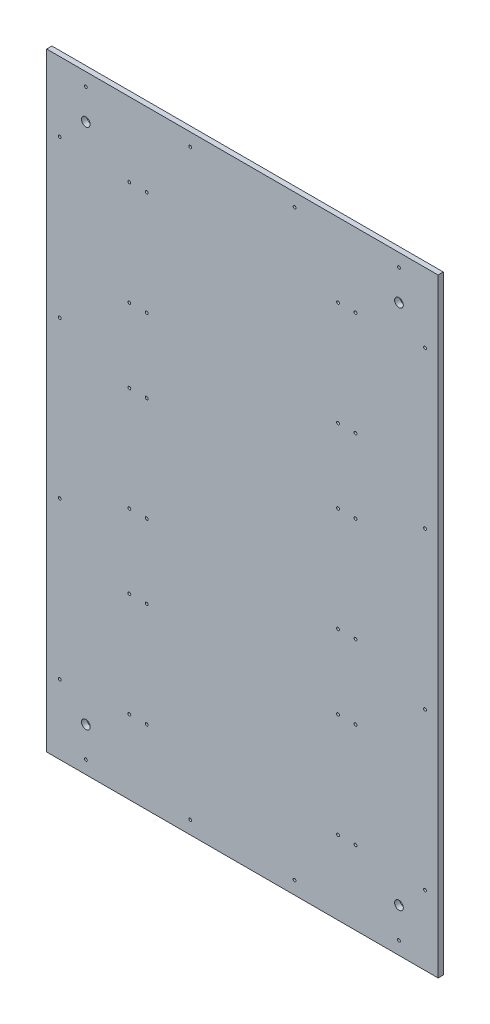
SolidWorks part; units mm, degrees
ref_plane "前视基准面" through (0, 0, 0) normal (0, 0, 1) x (1, 0, 0)
ref_plane "上视基准面" through (0, 0, 0) normal (0, 1, 0) x (1, 0, 0)
ref_plane "右视基准面" through (0, 0, 0) normal (1, 0, 0) x (0, 0, -1)
sketch "草图1" plane through (0, 0, 0) normal (0, 0, 1) x (1, 0, 0)
  line L1 (-225, 350) -> (225, 350)
  line L2 (-225, 350) -> (-225, -350)
  line L3 (-225, -350) -> (225, -350)
  line L4 (225, 350) -> (225, -350)
  line L5 (-225, 350) -> (225, -350) construction
  line L6 (-225, -350) -> (225, 350) construction
  point P0 (0, 0)
  dimension "D1" = 450
  dimension "D2" = 700
extrude "凸台-拉伸1" add sketch "草图1" along normal blind 6
hole_wizard "M4 螺纹孔1" positions "草图3" profile "草图2" tap size "M4" standard "Iso"
sketch "草图3" plane through (0, 0, 6) normal (0, 0, 1) x (1, 0, 0)
  point P0 (130, -265)
  point P3 (110, -265)
  point P6 (110, -145)
  point P9 (130, -145)
  point P12 (110, -60)
  point P15 (130, -60)
  point P18 (130, 60)
  point P21 (110, 60)
  point P25 (-130, -265)
  point P28 (-110, -265)
  point P31 (-130, -145)
  point P36 (-110, -145)
  point P38 (-130, -60)
  point P41 (-110, -60)
  point P44 (-130, 60)
  point P47 (-110, 60)
  point P50 (-130, 145)
  point P53 (-110, 145)
  point P56 (-130, 265)
  point P59 (-110, 265)
  point P67 (110, 145)
  point P70 (130, 145)
  point P73 (110, 265)
  point P76 (130, 265)
sketch "草图2" plane through (130, -265, 6) normal (1, 0, 0) x (0, -1, 0)
  line L0 (0, 0) -> (0, 28.0914)
  line L1 (0, 28.0914) -> (1.65, 27.1)
  line L2 (1.65, 27.1) -> (1.65, 0)
  line L5 (1.65, 0) -> (0, 0)
  line L10 (0, 28.0914) -> (-1.65, 27.1) construction
  line L11 (0, -6.35) -> (0, 107.95) construction
  dimension "螺纹孔钻头直径" = 3.3
  dimension "螺纹孔钻头深度" = 27.1
  dimension "导头角度" = 118
cosmetic thread "孔螺蚊线1" parameters "D1"=6, "D2"=4
cosmetic thread "孔螺蚊线2" parameters "D1"=6, "D2"=4
cosmetic thread "孔螺蚊线3" parameters "D1"=6, "D2"=4
cosmetic thread "孔螺蚊线4" parameters "D1"=6, "D2"=4
cosmetic thread "孔螺蚊线5" parameters "D1"=6, "D2"=4
cosmetic thread "孔螺蚊线6" parameters "D1"=6, "D2"=4
cosmetic thread "孔螺蚊线7" parameters "D1"=6, "D2"=4
cosmetic thread "孔螺蚊线8" parameters "D1"=6, "D2"=4
cosmetic thread "孔螺蚊线9" parameters "D1"=6, "D2"=4
cosmetic thread "孔螺蚊线10" parameters "D1"=6, "D2"=4
cosmetic thread "孔螺蚊线11" parameters "D1"=6, "D2"=4
cosmetic thread "孔螺蚊线12" parameters "D1"=6, "D2"=4
cosmetic thread "孔螺蚊线13" parameters "D1"=6, "D2"=4
cosmetic thread "孔螺蚊线14" parameters "D1"=6, "D2"=4
cosmetic thread "孔螺蚊线15" parameters "D1"=6, "D2"=4
cosmetic thread "孔螺蚊线16" parameters "D1"=6, "D2"=4
cosmetic thread "孔螺蚊线17" parameters "D1"=6, "D2"=4
cosmetic thread "孔螺蚊线18" parameters "D1"=6, "D2"=4
cosmetic thread "孔螺蚊线19" parameters "D1"=6, "D2"=4
cosmetic thread "孔螺蚊线20" parameters "D1"=6, "D2"=4
cosmetic thread "孔螺蚊线21" parameters "D1"=6, "D2"=4
cosmetic thread "孔螺蚊线22" parameters "D1"=6, "D2"=4
cosmetic thread "孔螺蚊线23" parameters "D1"=6, "D2"=4
cosmetic thread "孔螺蚊线24" parameters "D1"=6, "D2"=4
hole_wizard "M4 螺纹孔2" positions "草图6" profile "草图5" tap size "M4" standard "Iso"
sketch "草图6" plane through (0, 0, 6) normal (0, 0, 1) x (1, 0, 0)
  line L0 (-225, 0) -> (225, 0) construction
  line L1 (-225, 350) -> (-225, -350) construction
  line L2 (225, -350) -> (225, 350) construction
  line L4 (0, 350) -> (0, -350) construction
  line L5 (225, 350) -> (-225, 350) construction
  line L6 (-225, -350) -> (225, -350) construction
  point P0 (-180, 335)
  point P2 (-60, 335)
  point P4 (60, 335)
  point P6 (180, 335)
  point P8 (-180, -335)
  point P10 (-60, -335)
  point P12 (60, -335)
  point P14 (180, -335)
  point P16 (210, -270)
  point P18 (210, -90)
  point P20 (210, 90)
  point P22 (210, 270)
  point P24 (-210, 270)
  point P26 (-210, 90)
  point P28 (-210, -90)
  point P30 (-210, -270)
  dimension "D1" = 120
  dimension "D2" = 15
  dimension "D3" = 120
  dimension "D4" = 120
  dimension "D5" = 15
  dimension "D6" = 15
  dimension "D7" = 15
  dimension "D8" = 180
  dimension "D9" = 180
sketch "草图5" plane through (-180, 335, 6) normal (1, 0, 0) x (0, -1, 0)
  line L0 (0, 0) -> (0, 28.0914)
  line L1 (0, 28.0914) -> (1.65, 27.1)
  line L2 (1.65, 27.1) -> (1.65, 0)
  line L5 (1.65, 0) -> (0, 0)
  line L10 (0, 28.0914) -> (-1.65, 27.1) construction
  line L11 (0, -6.35) -> (0, 107.95) construction
  dimension "螺纹孔钻头直径" = 3.3
  dimension "螺纹孔钻头深度" = 27.1
  dimension "导头角度" = 118
cosmetic thread "孔螺蚊线25" parameters "D1"=6, "D2"=4
cosmetic thread "孔螺蚊线26" parameters "D1"=6, "D2"=4
cosmetic thread "孔螺蚊线27" parameters "D1"=6, "D2"=4
cosmetic thread "孔螺蚊线28" parameters "D1"=6, "D2"=4
cosmetic thread "孔螺蚊线29" parameters "D1"=6, "D2"=4
cosmetic thread "孔螺蚊线30" parameters "D1"=6, "D2"=4
cosmetic thread "孔螺蚊线31" parameters "D1"=6, "D2"=4
cosmetic thread "孔螺蚊线32" parameters "D1"=6, "D2"=4
cosmetic thread "孔螺蚊线33" parameters "D1"=6, "D2"=4
cosmetic thread "孔螺蚊线34" parameters "D1"=6, "D2"=4
cosmetic thread "孔螺蚊线35" parameters "D1"=6, "D2"=4
cosmetic thread "孔螺蚊线36" parameters "D1"=6, "D2"=4
cosmetic thread "孔螺蚊线37" parameters "D1"=6, "D2"=4
cosmetic thread "孔螺蚊线38" parameters "D1"=6, "D2"=4
cosmetic thread "孔螺蚊线39" parameters "D1"=6, "D2"=4
cosmetic thread "孔螺蚊线40" parameters "D1"=6, "D2"=4
sketch "草图7" plane through (0, 0, 6) normal (0, 0, 1) x (1, 0, 0)
  line L0 (0, 0) -> (0, -390.7084) construction
  line L1 (0, 0) -> (347.399, 0) construction
  circle A0 centre (180, -300) radius 5
  circle A1 centre (-180, -300) radius 5
  circle A2 centre (-180, 300) radius 5
  circle A3 centre (180, 300) radius 5
  dimension "D1" = 600
  dimension "D2" = 360
  dimension "D3" = 360
  dimension "D4" = 600
  dimension "D5" = 10
extrude "切除-拉伸1" cut sketch "草图7" against normal blind 10
